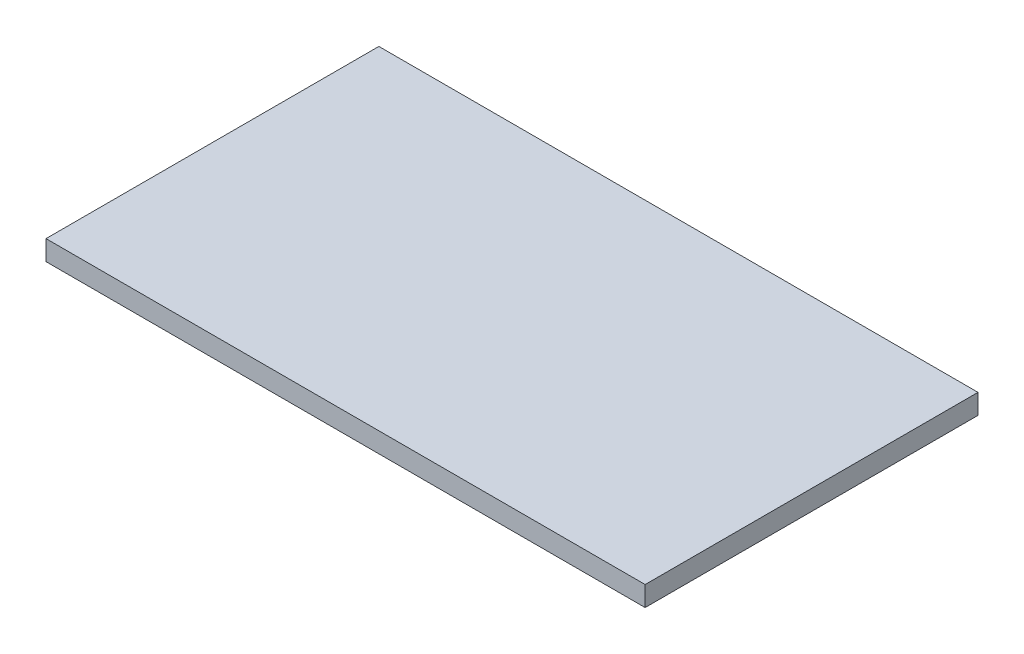
SolidWorks part; units mm, degrees
ref_plane "Front Plane" through (0, 0, 0) normal (0, 0, 1) x (1, 0, 0)
ref_plane "Top Plane" through (0, 0, 0) normal (0, 1, 0) x (1, 0, 0)
ref_plane "Right Plane" through (0, 0, 0) normal (1, 0, 0) x (0, 0, -1)
sketch "Sketch1" plane through (0, 0, 0) normal (0, 1, 0) x (1, 0, 0)
  line L1 (-90, 50) -> (90, 50)
  line L2 (-90, 50) -> (-90, -50)
  line L3 (-90, -50) -> (90, -50)
  line L4 (90, 50) -> (90, -50)
  line L5 (-90, 50) -> (90, -50) construction
  line L6 (-90, -50) -> (90, 50) construction
  point P0 (0, 0)
  dimension "D1" = 180
  dimension "D2" = 100
extrude "Boss-Extrude1" add sketch "Sketch1" along normal blind 6
